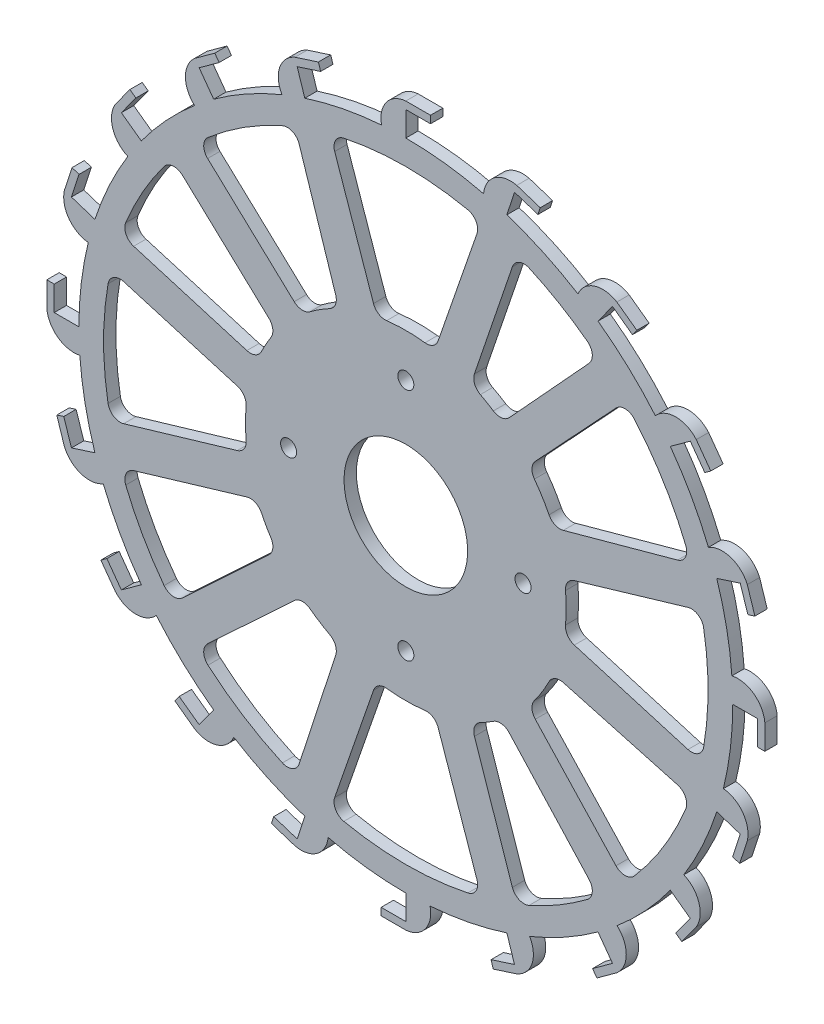
from build123d import *

# Parameters (mm, degrees)
SKETCH_1_R          = 15
SKETCH_1_R_2        = 3.25
EXTRUDE_1_DEPTH     = 5
EXTRUDE_3_DEPTH     = 5
FILLET_1_R          = 5
SKETCH_3_R          = 25.05
CUT_EXTRUDE_1_DEPTH = 206.828812366


with BuildPart() as part:
    # 草图1 → 凸台-拉伸1 (new body)
    with BuildSketch(Plane.XY):
        with BuildLine():
            Line((0, 145.5), (10, 145.5))
            Line((10, 145.5), (10, 142.5))
            Line((10, 142.5), (0, 142.5))
            Line((0, 142.5), (0, 132.5))
            ThreePointArc((0, 132.5), (15.863549131, 131.546941466), (31.498888588, 128.701476362))
            ThreePointArc((31.498888588, 128.701476362), (36.030071565, 136.601261654), (44.961972682, 138.378723121))
            Line((44.961972682, 138.378723121), (54.472537845, 135.288553177))
            Line((54.472537845, 135.288553177), (53.545486861, 132.435383628))
            Line((53.545486861, 132.435383628), (44.034921698, 135.525553572))
            Line((44.034921698, 135.525553572), (40.944751755, 126.014988409))
            ThreePointArc((40.944751755, 126.014988409), (55.737372243, 120.206469607), (69.728166645, 112.668685873))
            ThreePointArc((69.728166645, 112.668685873), (76.478745648, 118.781615608), (85.522754209, 117.711972682))
            Line((85.522754209, 117.711972682), (93.612924152, 111.834120159))
            Line((93.612924152, 111.834120159), (91.849568395, 109.407069176))
            Line((91.849568395, 109.407069176), (83.759398452, 115.284921698))
            Line((83.759398452, 115.284921698), (77.881545929, 107.194751755))
            ThreePointArc((77.881545929, 107.194751755), (90.155233016, 97.099350976), (101.131965925, 85.607099402))
            ThreePointArc((101.131965925, 85.607099402), (109.441147249, 89.334797426), (117.711972682, 85.522754209))
            Line((117.711972682, 85.522754209), (123.589825204, 77.432584265))
            Line((123.589825204, 77.432584265), (121.162774221, 75.669228508))
            Line((121.162774221, 75.669228508), (115.284921698, 83.759398452))
            Line((115.284921698, 83.759398452), (107.194751755, 77.881545929))
            ThreePointArc((107.194751755, 77.881545929), (115.748071432, 64.48747134), (122.636263754, 50.165693582))
            ThreePointArc((122.636263754, 50.165693582), (131.690686836, 51.14326684), (138.378723121, 44.961972682))
            Line((138.378723121, 44.961972682), (141.468893065, 35.451407519))
            Line((141.468893065, 35.451407519), (138.615723516, 34.524356535))
            Line((138.615723516, 34.524356535), (135.525553572, 44.034921698))
            Line((135.525553572, 44.034921698), (126.014988409, 40.944751755))
            ThreePointArc((126.014988409, 40.944751755), (130.010682152, 25.563108698), (132.136069628, 9.813720149))
            ThreePointArc((132.136069628, 9.813720149), (141.049424452, 7.94547696), (145.5, 0))
            Line((145.5, 0), (145.5, -10))
            Line((145.5, -10), (142.5, -10))
            Line((142.5, -10), (142.5, 0))
            Line((142.5, 0), (132.5, 0))
            ThreePointArc((132.5, 0), (131.546941466, -15.863549131), (128.701476362, -31.498888588))
            ThreePointArc((128.701476362, -31.498888588), (136.601261654, -36.030071565), (138.378723121, -44.961972682))
            Line((138.378723121, -44.961972682), (135.288553177, -54.472537845))
            Line((135.288553177, -54.472537845), (132.435383628, -53.545486861))
            Line((132.435383628, -53.545486861), (135.525553572, -44.034921698))
            Line((135.525553572, -44.034921698), (126.014988409, -40.944751755))
            ThreePointArc((126.014988409, -40.944751755), (120.206469607, -55.737372243), (112.668685873, -69.728166645))
            ThreePointArc((112.668685873, -69.728166645), (118.781615608, -76.478745648), (117.711972682, -85.522754209))
            Line((117.711972682, -85.522754209), (111.834120159, -93.612924152))
            Line((111.834120159, -93.612924152), (109.407069176, -91.849568395))
            Line((109.407069176, -91.849568395), (115.284921698, -83.759398452))
            Line((115.284921698, -83.759398452), (107.194751755, -77.881545929))
            ThreePointArc((107.194751755, -77.881545929), (97.099350976, -90.155233016), (85.607099402, -101.131965925))
            ThreePointArc((85.607099402, -101.131965925), (89.334797426, -109.441147249), (85.522754209, -117.711972682))
            Line((85.522754209, -117.711972682), (77.432584265, -123.589825204))
            Line((77.432584265, -123.589825204), (75.669228508, -121.162774221))
            Line((75.669228508, -121.162774221), (83.759398452, -115.284921698))
            Line((83.759398452, -115.284921698), (77.881545929, -107.194751755))
            ThreePointArc((77.881545929, -107.194751755), (64.48747134, -115.748071432), (50.165693582, -122.636263754))
            ThreePointArc((50.165693582, -122.636263754), (51.14326684, -131.690686836), (44.961972682, -138.378723121))
            Line((44.961972682, -138.378723121), (35.451407519, -141.468893065))
            Line((35.451407519, -141.468893065), (34.524356535, -138.615723516))
            Line((34.524356535, -138.615723516), (44.034921698, -135.525553572))
            Line((44.034921698, -135.525553572), (40.944751755, -126.014988409))
            ThreePointArc((40.944751755, -126.014988409), (25.563108698, -130.010682152), (9.813720149, -132.136069628))
            ThreePointArc((9.813720149, -132.136069628), (7.94547696, -141.049424452), (0, -145.5))
            Line((0, -145.5), (-10, -145.5))
            Line((-10, -145.5), (-10, -142.5))
            Line((-10, -142.5), (0, -142.5))
            Line((0, -142.5), (0, -132.5))
            ThreePointArc((0, -132.5), (-15.863549131, -131.546941466), (-31.498888588, -128.701476362))
            ThreePointArc((-31.498888588, -128.701476362), (-36.030071565, -136.601261654), (-44.961972682, -138.378723121))
            Line((-44.961972682, -138.378723121), (-54.472537845, -135.288553177))
            Line((-54.472537845, -135.288553177), (-53.545486861, -132.435383628))
            Line((-53.545486861, -132.435383628), (-44.034921698, -135.525553572))
            Line((-44.034921698, -135.525553572), (-40.944751755, -126.014988409))
            ThreePointArc((-40.944751755, -126.014988409), (-55.737372243, -120.206469607), (-69.728166645, -112.668685873))
            ThreePointArc((-69.728166645, -112.668685873), (-76.478745648, -118.781615608), (-85.522754209, -117.711972682))
            Line((-85.522754209, -117.711972682), (-93.612924152, -111.834120159))
            Line((-93.612924152, -111.834120159), (-91.849568395, -109.407069176))
            Line((-91.849568395, -109.407069176), (-83.759398452, -115.284921698))
            Line((-83.759398452, -115.284921698), (-77.881545929, -107.194751755))
            ThreePointArc((-77.881545929, -107.194751755), (-90.155233016, -97.099350976), (-101.131965925, -85.607099402))
            ThreePointArc((-101.131965925, -85.607099402), (-109.441147249, -89.334797426), (-117.711972682, -85.522754209))
            Line((-117.711972682, -85.522754209), (-123.589825204, -77.432584265))
            Line((-123.589825204, -77.432584265), (-121.162774221, -75.669228508))
            Line((-121.162774221, -75.669228508), (-115.284921698, -83.759398452))
            Line((-115.284921698, -83.759398452), (-107.194751755, -77.881545929))
            ThreePointArc((-107.194751755, -77.881545929), (-115.748071432, -64.48747134), (-122.636263754, -50.165693582))
            ThreePointArc((-122.636263754, -50.165693582), (-131.690686836, -51.14326684), (-138.378723121, -44.961972682))
            Line((-138.378723121, -44.961972682), (-141.468893065, -35.451407519))
            Line((-141.468893065, -35.451407519), (-138.615723516, -34.524356535))
            Line((-138.615723516, -34.524356535), (-135.525553572, -44.034921698))
            Line((-135.525553572, -44.034921698), (-126.014988409, -40.944751755))
            ThreePointArc((-126.014988409, -40.944751755), (-130.010682152, -25.563108698), (-132.136069628, -9.813720149))
            ThreePointArc((-132.136069628, -9.813720149), (-141.049424452, -7.94547696), (-145.5, 0))
            Line((-145.5, 0), (-145.5, 10))
            Line((-145.5, 10), (-142.5, 10))
            Line((-142.5, 10), (-142.5, 0))
            Line((-142.5, 0), (-132.5, 0))
            ThreePointArc((-132.5, 0), (-131.546941466, 15.863549131), (-128.701476362, 31.498888588))
            ThreePointArc((-128.701476362, 31.498888588), (-136.601261654, 36.030071565), (-138.378723121, 44.961972682))
            Line((-138.378723121, 44.961972682), (-135.288553177, 54.472537845))
            Line((-135.288553177, 54.472537845), (-132.435383628, 53.545486861))
            Line((-132.435383628, 53.545486861), (-135.525553572, 44.034921698))
            Line((-135.525553572, 44.034921698), (-126.014988409, 40.944751755))
            ThreePointArc((-126.014988409, 40.944751755), (-120.206469607, 55.737372243), (-112.668685873, 69.728166645))
            ThreePointArc((-112.668685873, 69.728166645), (-118.781615608, 76.478745648), (-117.711972682, 85.522754209))
            Line((-117.711972682, 85.522754209), (-111.834120159, 93.612924152))
            Line((-111.834120159, 93.612924152), (-109.407069176, 91.849568395))
            Line((-109.407069176, 91.849568395), (-115.284921698, 83.759398452))
            Line((-115.284921698, 83.759398452), (-107.194751755, 77.881545929))
            ThreePointArc((-107.194751755, 77.881545929), (-97.099350976, 90.155233016), (-85.607099402, 101.131965925))
            ThreePointArc((-85.607099402, 101.131965925), (-89.334797426, 109.441147249), (-85.522754209, 117.711972682))
            Line((-85.522754209, 117.711972682), (-77.432584265, 123.589825204))
            Line((-77.432584265, 123.589825204), (-75.669228508, 121.162774221))
            Line((-75.669228508, 121.162774221), (-83.759398452, 115.284921698))
            Line((-83.759398452, 115.284921698), (-77.881545929, 107.194751755))
            ThreePointArc((-77.881545929, 107.194751755), (-64.48747134, 115.748071432), (-50.165693582, 122.636263754))
            ThreePointArc((-50.165693582, 122.636263754), (-51.14326684, 131.690686836), (-44.961972682, 138.378723121))
            Line((-44.961972682, 138.378723121), (-35.451407519, 141.468893065))
            Line((-35.451407519, 141.468893065), (-34.524356535, 138.615723516))
            Line((-34.524356535, 138.615723516), (-44.034921698, 135.525553572))
            Line((-44.034921698, 135.525553572), (-40.944751755, 126.014988409))
            ThreePointArc((-40.944751755, 126.014988409), (-25.563108698, 130.010682152), (-9.813720149, 132.136069628))
            ThreePointArc((-9.813720149, 132.136069628), (-7.94547696, 141.049424452), (0, 145.5))
        make_face()
        Circle(SKETCH_1_R, mode=Mode.SUBTRACT)
        with Locations((47.5, 0)):
            Circle(SKETCH_1_R_2, mode=Mode.SUBTRACT)
        with Locations((0, -47.5)):
            Circle(SKETCH_1_R_2, mode=Mode.SUBTRACT)
        with Locations((-47.5, 0)):
            Circle(SKETCH_1_R_2, mode=Mode.SUBTRACT)
        with Locations((0, 47.5)):
            Circle(SKETCH_1_R_2, mode=Mode.SUBTRACT)
        with BuildLine():
            Line((115.4655256, -40.91408557), (25.295414942, -16.128917599))
            Line((25.295414942, -16.128917599), (88.873223604, -84.30777026))
            ThreePointArc((88.873223604, -84.30777026), (104.447757632, -64.00715527), (115.4655256, -40.91408557))
        make_face(mode=Mode.SUBTRACT)
        with BuildLine():
            Line((-30.646438581, 118.604577493), (-11.736248398, 63.93168599))
            ThreePointArc((-11.736248398, 63.93168599), (0, 65), (11.736248398, 63.93168599))
            Line((11.736248398, 63.93168599), (30.646438581, 118.604577493))
            ThreePointArc((30.646438581, 118.604577493), (0, 122.5), (-30.646438581, 118.604577493))
        make_face(mode=Mode.SUBTRACT)
        with BuildLine():
            Line((-119.601341953, -26.490923031), (-64.208340167, -10.113805068))
            ThreePointArc((-64.208340167, -10.113805068), (-65, 0), (-64.208340167, 10.113805068))
            Line((-64.208340167, 10.113805068), (-119.601341953, 26.490923031))
            ThreePointArc((-119.601341953, 26.490923031), (-122.5, 0), (-119.601341953, -26.490923031))
        make_face(mode=Mode.SUBTRACT)
        with BuildLine():
            Line((30.646438581, -118.604577493), (11.736248398, -63.93168599))
            ThreePointArc((11.736248398, -63.93168599), (0, -65), (-11.736248398, -63.93168599))
            Line((-11.736248398, -63.93168599), (-30.646438581, -118.604577493))
            ThreePointArc((-30.646438581, -118.604577493), (0, -122.5), (30.646438581, -118.604577493))
        make_face(mode=Mode.SUBTRACT)
        with BuildLine():
            Line((-115.467174059, 40.909433079), (-26.347643759, 14.345789221))
            Line((-26.347643759, 14.345789221), (-94.537709943, 77.902961425))
            ThreePointArc((-94.537709943, 77.902961425), (-106.619149832, 60.320866116), (-115.467174059, 40.909433079))
        make_face(mode=Mode.SUBTRACT)
        with BuildLine():
            Line((-94.537709943, -77.902961425), (-26.347643759, -14.345789221))
            Line((-26.347643759, -14.345789221), (-115.467174059, -40.909433079))
            ThreePointArc((-115.467174059, -40.909433079), (-106.619149832, -60.320866116), (-94.537709943, -77.902961425))
        make_face(mode=Mode.SUBTRACT)
        with BuildLine():
            Line((-44.916491293, -113.968235969), (-16.109056419, -25.308067909))
            Line((-16.109056419, -25.308067909), (-84.307729511, -88.87326226))
            ThreePointArc((-84.307729511, -88.87326226), (-65.819178337, -103.315467201), (-44.916491293, -113.968235969))
        make_face(mode=Mode.SUBTRACT)
        with BuildLine():
            Line((77.904348966, -94.536566535), (15, -25.980762114))
            Line((15, -25.980762114), (44.913590331, -113.969379237))
            ThreePointArc((44.913590331, -113.969379237), (62.172904916, -105.549892915), (77.904348966, -94.536566535))
        make_face(mode=Mode.SUBTRACT)
        with BuildLine():
            Line((88.873223604, 84.30777026), (25.295414942, 16.128917599))
            Line((25.295414942, 16.128917599), (115.4655256, 40.91408557))
            ThreePointArc((115.4655256, 40.91408557), (104.447757632, 64.00715527), (88.873223604, 84.30777026))
        make_face(mode=Mode.SUBTRACT)
        with BuildLine():
            Line((119.601341953, 26.490923031), (64.208340167, 10.113805068))
            ThreePointArc((64.208340167, 10.113805068), (65, 0), (64.208340167, -10.113805068))
            Line((64.208340167, -10.113805068), (119.601341953, -26.490923031))
            ThreePointArc((119.601341953, -26.490923031), (122.5, 0), (119.601341953, 26.490923031))
        make_face(mode=Mode.SUBTRACT)
        with BuildLine():
            Line((44.913590331, 113.969379237), (15, 25.980762114))
            Line((15, 25.980762114), (77.904348966, 94.536566535))
            ThreePointArc((77.904348966, 94.536566535), (62.172904916, 105.549892915), (44.913590331, 113.969379237))
        make_face(mode=Mode.SUBTRACT)
        with BuildLine():
            Line((-84.307729511, 88.87326226), (-16.109056419, 25.308067909))
            Line((-16.109056419, 25.308067909), (-44.916491293, 113.968235969))
            ThreePointArc((-44.916491293, 113.968235969), (-65.819178337, 103.315467201), (-84.307729511, 88.87326226))
        make_face(mode=Mode.SUBTRACT)
    extrude(amount=EXTRUDE_1_DEPTH)

    # 草图2 → 凸台-拉伸3 (add, through all)
    with BuildSketch(Plane.XY.offset(5)):
        with BuildLine():
            Line((-42.094650671, 49.528177686), (-16.109056419, 25.308067909))
            Line((-16.109056419, 25.308067909), (-27.084871204, 59.088152381))
            ThreePointArc((-27.084871204, 59.088152381), (-34.918474204, 54.824266153), (-42.094650671, 49.528177686))
        make_face()
        with BuildLine():
            Line((-60.228430136, 24.444553655), (-26.347643759, 14.345789221))
            Line((-26.347643759, 14.345789221), (-52.327027932, 38.560110838))
            ThreePointArc((-52.327027932, 38.560110838), (-56.718559783, 31.7490941), (-60.228430136, 24.444553655))
        make_face()
        with BuildLine():
            Line((15, -25.980762114), (26.365821175, -59.412485841))
            ThreePointArc((26.365821175, -59.412485841), (32.852239745, -56.086810782), (38.925507456, -52.055786127))
            Line((38.925507456, -52.055786127), (15, -25.980762114))
        make_face()
        with BuildLine():
            Line((25.295414942, -16.128917599), (49.518961932, -42.105491437))
            ThreePointArc((49.518961932, -42.105491437), (55.252901221, -34.236192934), (59.747031858, -25.598675437))
            Line((59.747031858, -25.598675437), (25.295414942, -16.128917599))
        make_face()
        with BuildLine():
            Line((25.295414942, 16.128917599), (59.747031858, 25.598675437))
            ThreePointArc((59.747031858, 25.598675437), (55.252901221, 34.236192934), (49.518961932, 42.105491437))
            Line((49.518961932, 42.105491437), (25.295414942, 16.128917599))
        make_face()
        with BuildLine():
            Line((15, 25.980762114), (38.925507456, 52.055786127))
            ThreePointArc((38.925507456, 52.055786127), (32.852239745, 56.086810782), (26.365821175, 59.412485841))
            Line((26.365821175, 59.412485841), (15, 25.980762114))
        make_face()
        with BuildLine():
            Line((-26.347643759, -14.345789221), (-60.228430136, -24.444553655))
            ThreePointArc((-60.228430136, -24.444553655), (-56.718559783, -31.7490941), (-52.327027932, -38.560110838))
            Line((-52.327027932, -38.560110838), (-26.347643759, -14.345789221))
        make_face()
        with BuildLine():
            Line((-16.109056419, -25.308067909), (-42.094650671, -49.528177686))
            ThreePointArc((-42.094650671, -49.528177686), (-34.918474204, -54.824266153), (-27.084871204, -59.088152381))
            Line((-27.084871204, -59.088152381), (-16.109056419, -25.308067909))
        make_face()
    extrude(amount=-EXTRUDE_3_DEPTH)

    # 圆角1
    fillet_1_edges = [part.edges().sort_by_distance(p)[0] for p in [
        (88.873223604, -84.30777026, 2.5),
        (115.4655256, -40.91408557, 2.5),
        (30.646438581, 118.604577493, 2.5),
        (-30.646438581, 118.604577493, 2.5),
        (-11.736248398, 63.93168599, 2.5),
        (11.736248398, 63.93168599, 2.5),
        (-119.601341953, 26.490923031, 2.5),
        (-119.601341953, -26.490923031, 2.5),
        (-64.208340167, -10.113805068, 2.5),
        (-64.208340167, 10.113805068, 2.5),
        (-30.646438581, -118.604577493, 2.5),
        (30.646438581, -118.604577493, 2.5),
        (11.736248398, -63.93168599, 2.5),
        (-11.736248398, -63.93168599, 2.5),
        (-94.537709943, 77.902961425, 2.5),
        (-115.467174059, 40.909433079, 2.5),
        (-115.467174059, -40.909433079, 2.5),
        (-94.537709943, -77.902961425, 2.5),
        (-84.307729511, -88.87326226, 2.5),
        (-44.916491293, -113.968235969, 2.5),
        (44.913590331, -113.969379237, 2.5),
        (77.904348966, -94.536566535, 2.5),
        (115.4655256, 40.91408557, 2.5),
        (88.873223604, 84.30777026, 2.5),
        (119.601341953, -26.490923031, 2.5),
        (119.601341953, 26.490923031, 2.5),
        (64.208340167, 10.113805068, 2.5),
        (64.208340167, -10.113805068, 2.5),
        (77.904348966, 94.536566535, 2.5),
        (44.913590331, 113.969379237, 2.5),
        (-44.916491293, 113.968235969, 2.5),
        (-84.307729511, 88.87326226, 2.5),
        (-27.084871204, 59.088152381, 2.5),
        (-42.094650671, 49.528177686, 2.5),
        (38.925507456, -52.055786127, 2.5),
        (26.365821175, -59.412485841, 2.5),
        (-52.327027932, 38.560110838, 2.5),
        (-60.228430136, 24.444553655, 2.5),
        (-52.327027932, -38.560110838, 2.5),
        (-60.228430136, -24.444553655, 2.5),
        (59.747031858, -25.598675437, 2.5),
        (49.518961932, -42.105491437, 2.5),
        (49.518961932, 42.105491437, 2.5),
        (59.747031858, 25.598675437, 2.5),
        (26.365821175, 59.412485841, 2.5),
        (38.925507456, 52.055786127, 2.5),
        (-27.084871204, -59.088152381, 2.5),
        (-42.094650671, -49.528177686, 2.5),
    ]]
    fillet(fillet_1_edges, radius=FILLET_1_R)

    # 草图3 → 切除-拉伸1 (cut, through all)
    with BuildSketch(Plane(origin=(0, 0, 0), x_dir=(-1, 0, 0), z_dir=(0, 0, -1))):
        Circle(SKETCH_3_R)
    extrude(amount=-CUT_EXTRUDE_1_DEPTH, mode=Mode.SUBTRACT)


solid = part.part
